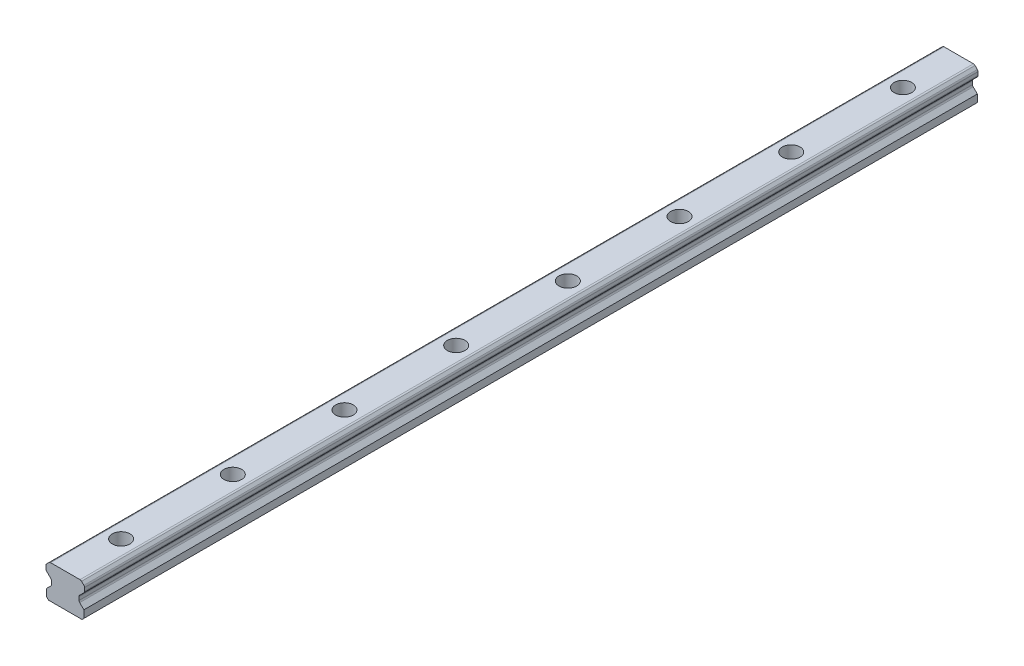
SolidWorks part; units mm, degrees
material "普通碳钢"
ref_plane "Front Plane" through (0, 0, 0) normal (0, 0, 1) x (1, 0, 0)
ref_plane "Top Plane" through (0, 0, 0) normal (0, 1, 0) x (1, 0, 0)
ref_plane "Right Plane" through (0, 0, 0) normal (1, 0, 0) x (0, 0, -1)
sketch "Sketch1" plane through (0, 0, 0) normal (0, 1, 0) x (1, 0, 0)
  line L1 (0, -48.5) -> (0, 48.5) construction
  line L2 (-22, -35.7) -> (22, -35.7)
  line L3 (-22, -35.7) -> (-22, 35.7)
  line L4 (-22, 35.7) -> (22, 35.7)
  line L5 (22, -35.7) -> (22, 35.7)
  line L6 (-22, 0) -> (22, 0) construction
  line L7 (22, -35.7) -> (22, -42) construction
  line L8 (0, -48.5) -> (0, -60.5) construction
  line L9 (22, 35.7) -> (22, 42) construction
  point P9 (-20, 20)
  point P12 (20, 20)
  point P13 (20, -20)
  point P14 (-20, -20)
  dimension "W" = 44
  dimension "L1" = 71.4
  dimension "L0" = 97
  dimension "B" = 40
  dimension "C" = 40
  dimension "K" = 6.5
  dimension "L2" = 12
sketch "Sketch2" plane through (0, 0, 0) normal (0, 0, 1) x (1, 0, 0)
  line L0 (-22, 0) -> (22, 0) construction
  line L1 (-22, 0) -> (22, 0)
  line L2 (-22, 0) -> (-22, 25)
  line L3 (-22, 25) -> (22, 25)
  line L4 (22, 0) -> (22, 25)
  line L5 (0, 0) -> (0, 25) construction
  line L7 (-10, -5) -> (10, -5)
  line L8 (-22, 21.1) -> (22, 21.1)
  line L9 (-10, -5) -> (-10, 0)
  line L10 (-10, 0) -> (-7.7627, 2.2373)
  line L11 (-7.4113, 3.0858) -> (-7.4113, 4.8515)
  line L12 (-7.7627, 5.7) -> (-10, 7.9373)
  line L13 (-10.3515, 8.7858) -> (-10.3515, 10.5515)
  line L14 (-10, 11.4) -> (-8.7515, 12.6485)
  line L15 (-7.9029, 13) -> (7.9029, 13)
  line L16 (10.3515, 8.7858) -> (10.3515, 10.5515)
  line L17 (7.7627, 5.7) -> (10, 7.9373)
  line L18 (7.4113, 3.0858) -> (7.4113, 4.8515)
  line L19 (10, 0) -> (7.7627, 2.2373)
  line L20 (10, 11.4) -> (8.7515, 12.6485)
  line L21 (10, -5) -> (10, 0)
  line L22 (-10, -5) -> (-22, -5) construction
  arc A0 (-7.7627, 2.2373) -> (-7.4113, 3.0858) centre (-8.6113, 3.0858) ccw
  arc A1 (-7.7627, 5.7) -> (-7.4113, 4.8515) centre (-8.6113, 4.8515) cw
  arc A2 (-10.3515, 8.7858) -> (-10, 7.9373) centre (-9.1515, 8.7858) ccw
  arc A3 (-10.3515, 10.5515) -> (-10, 11.4) centre (-9.1515, 10.5515) cw
  arc A4 (-8.7515, 12.6485) -> (-7.9029, 13) centre (-7.9029, 11.8) cw
  arc A5 (10.3515, 10.5515) -> (10, 11.4) centre (9.1515, 10.5515) ccw
  arc A6 (10.3515, 8.7858) -> (10, 7.9373) centre (9.1515, 8.7858) cw
  arc A7 (7.7627, 5.7) -> (7.4113, 4.8515) centre (8.6113, 4.8515) ccw
  arc A8 (7.7627, 2.2373) -> (7.4113, 3.0858) centre (8.6113, 3.0858) cw
  arc A9 (8.7515, 12.6485) -> (7.9029, 13) centre (7.9029, 11.8) ccw
  circle A10 centre (22, 15) radius 1.65
  point P9 (-22, 13.3)
  point P33 (-8.4, 13)
  point P50 (0, 13)
  dimension "D6" = 1.2
  dimension "(d1)" = 3.3
  dimension "D1" = 3.9
  dimension "H2" = 5
  dimension "H" = 30
  dimension "T" = 11.7
  dimension "D2" = 45
  dimension "W1" = 20
  dimension "D3" = 135
  dimension "H1" = 18
  dimension "D4" = 8.4
  dimension "D5" = 135
  dimension "N" = 10
  dimension "W2" = 12
sketch "Sketch3" plane through (0, 0, 0) normal (0, 0, 1) x (1, 0, 0)
  line L0 (-10, -5) -> (10, -5) construction
  line L1 (-10, -5) -> (-10, 0) construction
  line L2 (-10, 0) -> (-7.7627, 2.2373) construction
  line L3 (-7.4113, 3.0858) -> (-7.4113, 4.8515) construction
  line L4 (-7.7627, 5.7) -> (-10, 7.9373) construction
  line L5 (-10.3515, 8.7858) -> (-10.3515, 10.5515) construction
  line L6 (-10, 11.4) -> (-8.7515, 12.6485) construction
  line L7 (-7.9029, 13) -> (7.9029, 13) construction
  line L8 (10, 11.4) -> (8.7515, 12.6485) construction
  line L9 (10.3515, 8.7858) -> (10.3515, 10.5515) construction
  line L10 (7.7627, 5.7) -> (10, 7.9373) construction
  line L11 (7.4113, 3.0858) -> (7.4113, 4.8515) construction
  line L12 (10, 0) -> (7.7627, 2.2373) construction
  line L13 (10, -5) -> (10, 0) construction
  line L14 (-10, -5) -> (10, -5)
  line L15 (-10, -5) -> (-10, 0)
  line L16 (-10, 0) -> (-7.7627, 2.2373)
  line L17 (-7.4113, 3.0858) -> (-7.4113, 4.8515)
  line L18 (-7.7627, 5.7) -> (-10, 7.9373)
  line L19 (-10.3515, 8.7858) -> (-10.3515, 10.5515)
  line L20 (-10, 11.4) -> (-8.7515, 12.6485)
  line L21 (-7.9029, 13) -> (7.9029, 13)
  line L22 (10, 11.4) -> (8.7515, 12.6485)
  line L23 (10.3515, 8.7858) -> (10.3515, 10.5515)
  line L24 (7.7627, 5.7) -> (10, 7.9373)
  line L25 (7.4113, 3.0858) -> (7.4113, 4.8515)
  line L26 (10, 0) -> (7.7627, 2.2373)
  line L27 (10, -5) -> (10, 0)
  arc A0 (-7.7627, 2.2373) -> (-7.4113, 3.0858) centre (-8.6113, 3.0858) ccw construction
  arc A1 (-7.4113, 4.8515) -> (-7.7627, 5.7) centre (-8.6113, 4.8515) ccw construction
  arc A2 (-10.3515, 8.7858) -> (-10, 7.9373) centre (-9.1515, 8.7858) ccw construction
  arc A3 (-10, 11.4) -> (-10.3515, 10.5515) centre (-9.1515, 10.5515) ccw construction
  arc A4 (-7.9029, 13) -> (-8.7515, 12.6485) centre (-7.9029, 11.8) ccw construction
  arc A5 (8.7515, 12.6485) -> (7.9029, 13) centre (7.9029, 11.8) ccw construction
  arc A6 (10.3515, 10.5515) -> (10, 11.4) centre (9.1515, 10.5515) ccw construction
  arc A7 (10, 7.9373) -> (10.3515, 8.7858) centre (9.1515, 8.7858) ccw construction
  arc A8 (7.7627, 5.7) -> (7.4113, 4.8515) centre (8.6113, 4.8515) ccw construction
  arc A9 (7.4113, 3.0858) -> (7.7627, 2.2373) centre (8.6113, 3.0858) ccw construction
  arc A10 (-7.7627, 2.2373) -> (-7.4113, 3.0858) centre (-8.6113, 3.0858) ccw
  arc A11 (-7.4113, 4.8515) -> (-7.7627, 5.7) centre (-8.6113, 4.8515) ccw
  arc A12 (-10.3515, 8.7858) -> (-10, 7.9373) centre (-9.1515, 8.7858) ccw
  arc A13 (-10, 11.4) -> (-10.3515, 10.5515) centre (-9.1515, 10.5515) ccw
  arc A14 (-7.9029, 13) -> (-8.7515, 12.6485) centre (-7.9029, 11.8) ccw
  arc A15 (8.7515, 12.6485) -> (7.9029, 13) centre (7.9029, 11.8) ccw
  arc A16 (10.3515, 10.5515) -> (10, 11.4) centre (9.1515, 10.5515) ccw
  arc A17 (10, 7.9373) -> (10.3515, 8.7858) centre (9.1515, 8.7858) ccw
  arc A18 (7.7627, 5.7) -> (7.4113, 4.8515) centre (8.6113, 4.8515) ccw
  arc A19 (7.4113, 3.0858) -> (7.7627, 2.2373) centre (8.6113, 3.0858) ccw
extrude "Boss-Extrude1" add sketch "Sketch3" against normal blind 480
sketch "Sketch4" plane through (0, 0, 0) normal (0, 1, 0) x (1, 0, 0)
  line L0 (0, 0) -> (0, 480) construction
  line L1 (7.9029, 480) -> (-7.9029, 480) construction
  point P5 (0, 40)
  dimension "标准端距E" = 40
hole_wizard "Countersink Hole1" positions "Sketch6" profile "Sketch5" counterbore size "M6" standard "ISO" end condition through all
sketch "Sketch6" plane through (0, 13, 0) normal (0, 1, 0) x (-1, 0, 0)
  line L0 (-7.9029, 0) -> (7.9029, 0) construction
  point P0 (0, -30)
  dimension "D1" = 30
sketch "Sketch5" plane through (0, 13, -30) normal (1, 0, 0) x (0, 0, 1)
  line L0 (0, 0) -> (0, 18)
  line L1 (0, 18) -> (3, 18)
  line L3 (3, 18) -> (3, 8.5)
  line L4 (3, 8.5) -> (4.75, 8.5)
  line L5 (4.75, 8.5) -> (4.75, 0)
  line L7 (4.75, 0) -> (0, 0)
  line L11 (0, -6.35) -> (0, 107.95) construction
  dimension "(d)" = 6
  dimension "通孔孔深度" = 18
  dimension "D" = 9.5
  dimension "(h)" = 8.5
pattern_linear "LPattern1" count 8 spacing 60 along (0, 0, -1) of "Countersink Hole1"
chamfer "Chamfer1" distance 1 angle 45 2 edges at (-10, -5, -240) (10, -5, -240)
